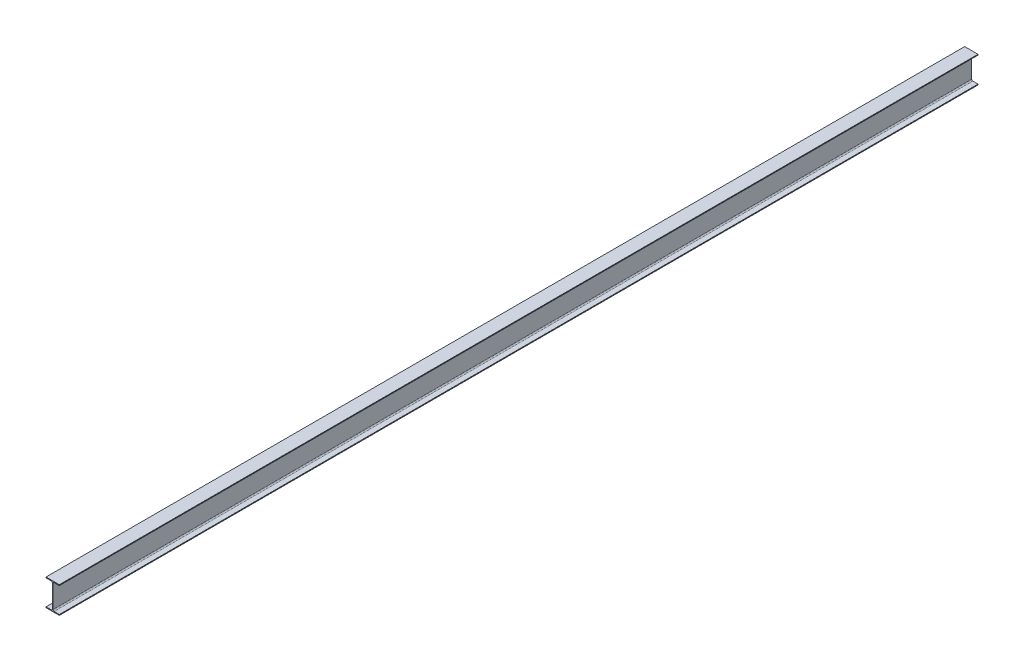
from build123d import *

# Parameters (mm, degrees)
BOSS_EXTRUDE1_DEPTH = 10347


with BuildPart() as part:
    # Sketch1 → Boss-Extrude1 (new body)
    with BuildSketch(Plane.XY):
        with BuildLine():
            Line((75, 0), (-75, 0))
            Line((-75, 0), (-75, 9))
            Line((-75, 9), (-16.25, 9))
            ThreePointArc((-16.25, 9), (-7.057611845, 12.807611845), (-3.25, 22))
            Line((-3.25, 22), (-3.25, 278))
            ThreePointArc((-3.25, 278), (-7.057611845, 287.192388155), (-16.25, 291))
            Line((-16.25, 291), (-75, 291))
            Line((-75, 291), (-75, 300))
            Line((-75, 300), (75, 300))
            Line((75, 300), (75, 291))
            Line((75, 291), (16.25, 291))
            ThreePointArc((16.25, 291), (7.057611845, 287.192388155), (3.25, 278))
            Line((3.25, 278), (3.25, 22))
            ThreePointArc((3.25, 22), (7.057611845, 12.807611845), (16.25, 9))
            Line((16.25, 9), (75, 9))
            Line((75, 9), (75, 0))
        make_face()
    extrude(amount=BOSS_EXTRUDE1_DEPTH)


solid = part.part
